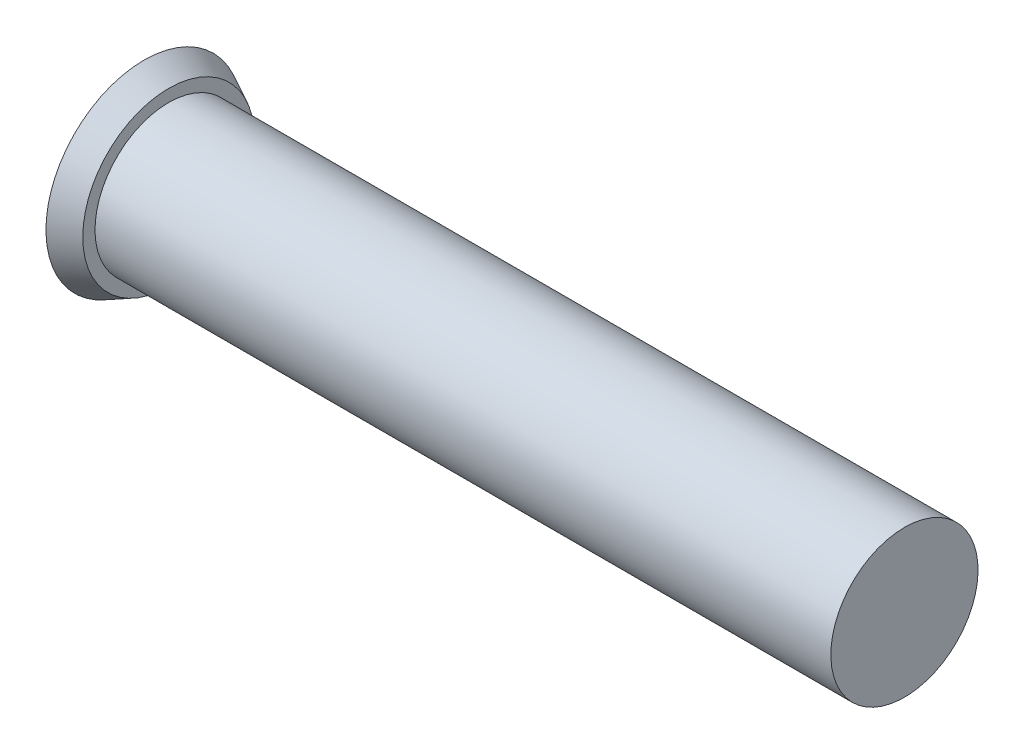
from build123d import *


with BuildPart() as part:
    # Sketch1 → Revolve1 (revolve)
    with BuildSketch(Plane.XY):
        Polygon((0, 0), (0, 4), (1, 3.5), (1, 3), (31, 3), (31, 0), align=None)
    revolve(axis=Axis((31, 0, 0), (-1, 0, 0)))


solid = part.part
